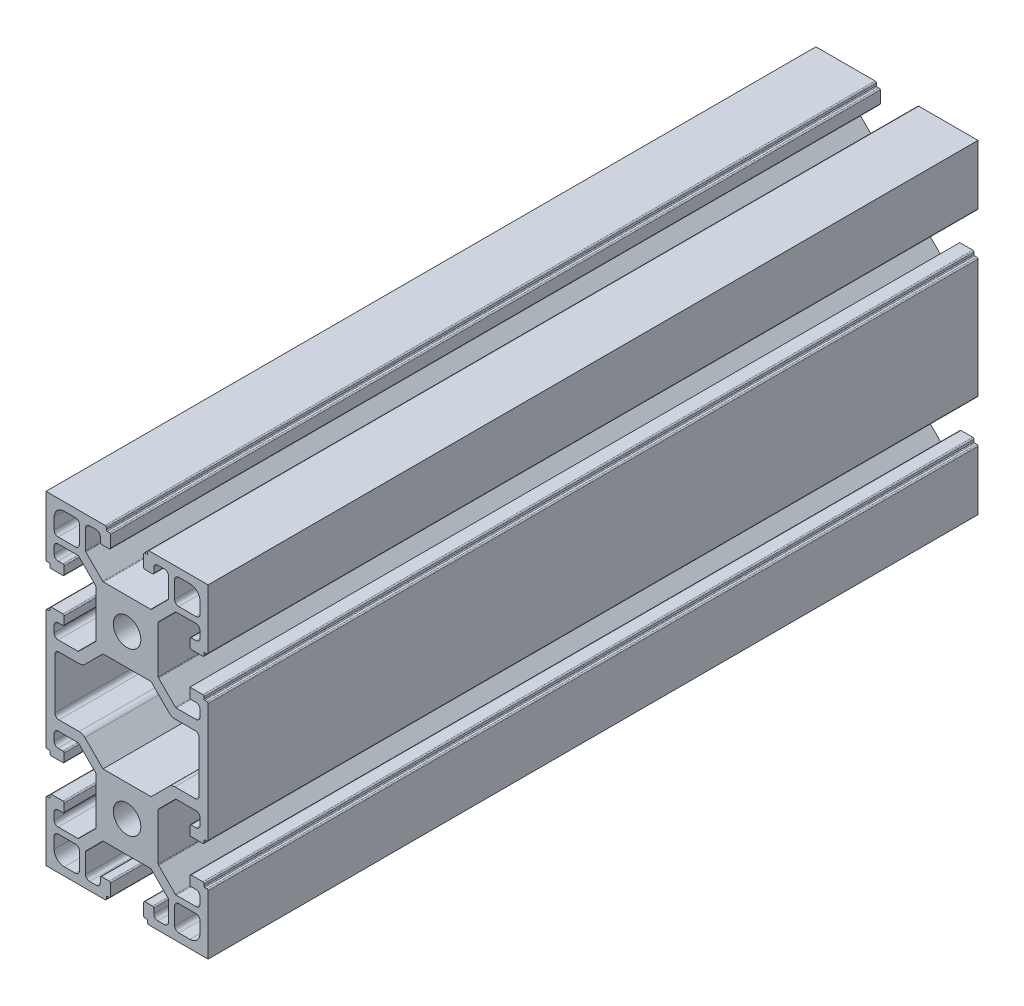
SolidWorks part; units mm, degrees
material "6061 合金"
ref_plane "前视基准面" through (0, 0, 0) normal (0, 0, 1) x (1, 0, 0)
ref_plane "上视基准面" through (0, 0, 0) normal (0, 1, 0) x (1, 0, 0)
ref_plane "右视基准面" through (0, 0, 0) normal (1, 0, 0) x (0, 0, -1)
sketch "Model" plane through (0, 0, 0) normal (0, 0, 1) x (1, 0, 0)
  line L0 (714.4099, 268.2298) -> (714.4099, 266.3298)
  line L1 (712.9099, 268.5298) -> (714.1099, 268.5298)
  line L2 (711.9099, 271.1798) -> (711.9099, 269.5298)
  line L3 (717.7679, 272.1798) -> (712.9099, 272.1798)
  line L4 (722.1221, 267.9499) -> (717.98, 272.0919)
  line L5 (722.2099, 256.1218) -> (722.2099, 267.7378)
  line L6 (717.98, 251.7677) -> (722.1221, 255.9097)
  line L7 (712.9099, 251.6798) -> (717.7679, 251.6798)
  line L8 (711.9099, 254.3298) -> (711.9099, 252.6798)
  line L9 (714.1099, 255.3298) -> (712.9099, 255.3298)
  line L10 (714.4099, 257.5298) -> (714.4099, 255.6298)
  line L11 (711.2099, 257.8298) -> (714.1099, 257.8298)
  line L12 (710.9099, 257.0298) -> (710.9099, 257.5298)
  line L13 (710.2099, 256.8298) -> (710.7099, 256.8298)
  line L14 (709.9099, 241.9298) -> (709.9099, 256.5298)
  line L15 (709.9099, 227.3298) -> (709.9099, 241.9298)
  line L16 (710.7099, 227.0298) -> (710.2099, 227.0298)
  line L17 (710.9099, 226.3298) -> (710.9099, 226.8298)
  line L18 (714.1099, 226.0298) -> (711.2099, 226.0298)
  line L19 (714.4099, 228.2298) -> (714.4099, 226.3298)
  line L20 (712.9099, 228.5298) -> (714.1099, 228.5298)
  line L21 (711.9099, 231.1798) -> (711.9099, 229.5298)
  line L22 (717.7679, 232.1798) -> (712.9099, 232.1798)
  line L23 (722.1221, 227.9499) -> (717.98, 232.0919)
  line L24 (722.2099, 216.1218) -> (722.2099, 227.7378)
  line L25 (717.98, 211.7677) -> (722.1221, 215.9097)
  line L26 (712.9099, 211.6798) -> (717.7679, 211.6798)
  line L27 (711.9099, 214.3298) -> (711.9099, 212.6798)
  line L28 (714.1099, 215.3298) -> (712.9099, 215.3298)
  line L29 (714.4099, 217.5298) -> (714.4099, 215.6298)
  line L30 (711.2099, 217.8298) -> (714.1099, 217.8298)
  line L31 (710.9099, 217.0298) -> (710.9099, 217.5298)
  line L32 (710.2099, 216.8298) -> (710.7099, 216.8298)
  line L33 (709.9099, 201.9298) -> (709.9099, 216.5298)
  line L34 (724.5099, 201.9298) -> (709.9099, 201.9298)
  line L35 (724.8099, 202.7298) -> (724.8099, 202.2298)
  line L36 (725.5099, 202.9298) -> (725.0099, 202.9298)
  line L37 (725.8099, 206.1298) -> (725.8099, 203.2298)
  line L38 (723.6099, 206.4298) -> (725.5099, 206.4298)
  line L39 (723.3099, 204.9298) -> (723.3099, 206.1298)
  line L40 (720.6599, 203.9298) -> (722.3099, 203.9298)
  line L41 (719.6599, 209.7878) -> (719.6599, 204.9298)
  line L42 (723.8898, 214.1419) -> (719.7478, 209.9999)
  line L43 (735.7179, 214.2298) -> (724.1019, 214.2298)
  line L44 (740.0721, 209.9999) -> (735.93, 214.1419)
  line L45 (740.1599, 204.9298) -> (740.1599, 209.7878)
  line L46 (737.5099, 203.9298) -> (739.1599, 203.9298)
  line L47 (736.5099, 206.1298) -> (736.5099, 204.9298)
  line L48 (734.3099, 206.4298) -> (736.2099, 206.4298)
  line L49 (734.0099, 203.2298) -> (734.0099, 206.1298)
  line L50 (734.8099, 202.9298) -> (734.3099, 202.9298)
  line L51 (735.0099, 202.2298) -> (735.0099, 202.7298)
  line L52 (749.9099, 201.9298) -> (735.3099, 201.9298)
  line L53 (749.9099, 216.5298) -> (749.9099, 201.9298)
  line L54 (749.1099, 216.8298) -> (749.6099, 216.8298)
  line L55 (748.9099, 217.5298) -> (748.9099, 217.0298)
  line L56 (745.7099, 217.8298) -> (748.6099, 217.8298)
  line L57 (745.4099, 215.6298) -> (745.4099, 217.5298)
  line L58 (746.9099, 215.3298) -> (745.7099, 215.3298)
  line L59 (747.9099, 212.6798) -> (747.9099, 214.3298)
  line L60 (742.0519, 211.6798) -> (746.9099, 211.6798)
  line L61 (737.6978, 215.9097) -> (741.8398, 211.7677)
  line L62 (737.6099, 227.7378) -> (737.6099, 216.1218)
  line L63 (741.8398, 232.0919) -> (737.6978, 227.9499)
  line L64 (746.9099, 232.1798) -> (742.0519, 232.1798)
  line L65 (747.9099, 229.5298) -> (747.9099, 231.1798)
  line L66 (745.7099, 228.5298) -> (746.9099, 228.5298)
  line L67 (745.4099, 226.3298) -> (745.4099, 228.2298)
  line L68 (748.6099, 226.0298) -> (745.7099, 226.0298)
  line L69 (748.9099, 226.8298) -> (748.9099, 226.3298)
  line L70 (749.6099, 227.0298) -> (749.1099, 227.0298)
  line L71 (749.9099, 241.9298) -> (749.9099, 227.3298)
  line L72 (749.9099, 256.5298) -> (749.9099, 241.9298)
  line L73 (749.1099, 256.8298) -> (749.6099, 256.8298)
  line L74 (748.9099, 257.5298) -> (748.9099, 257.0298)
  line L75 (745.4099, 257.8298) -> (748.6099, 257.8298)
  line L76 (745.4099, 255.3298) -> (745.4099, 257.8298)
  line L77 (746.9099, 255.3298) -> (745.4099, 255.3298)
  line L78 (747.9099, 252.6798) -> (747.9099, 254.3298)
  line L79 (742.0519, 251.6798) -> (746.9099, 251.6798)
  line L80 (737.6978, 255.9097) -> (741.8398, 251.7677)
  line L81 (737.6099, 267.7378) -> (737.6099, 256.1218)
  line L82 (741.8398, 272.0919) -> (737.6978, 267.9499)
  line L83 (746.9099, 272.1798) -> (742.0519, 272.1798)
  line L84 (747.9099, 269.5298) -> (747.9099, 271.1798)
  line L85 (745.7099, 268.5298) -> (746.9099, 268.5298)
  line L86 (745.4099, 266.3298) -> (745.4099, 268.2298)
  line L87 (748.6099, 266.0298) -> (745.7099, 266.0298)
  line L88 (748.9099, 266.8298) -> (748.9099, 266.3298)
  line L89 (749.6099, 267.0298) -> (749.1099, 267.0298)
  line L90 (749.9099, 281.9298) -> (749.9099, 267.3298)
  line L91 (735.3099, 281.9298) -> (749.9099, 281.9298)
  line L92 (735.0099, 281.1298) -> (735.0099, 281.6298)
  line L93 (734.3099, 280.9298) -> (734.8099, 280.9298)
  line L94 (734.0099, 277.7298) -> (734.0099, 280.6298)
  line L95 (736.2099, 277.4298) -> (734.3099, 277.4298)
  line L96 (736.5099, 278.9298) -> (736.5099, 277.7298)
  line L97 (739.1599, 279.9298) -> (737.5099, 279.9298)
  line L98 (740.1599, 274.0718) -> (740.1599, 278.9298)
  line L99 (735.93, 269.7177) -> (740.0721, 273.8597)
  line L100 (724.1019, 269.6298) -> (735.7179, 269.6298)
  line L101 (719.7478, 273.8597) -> (723.8898, 269.7177)
  line L102 (719.6599, 278.9298) -> (719.6599, 274.0718)
  line L103 (722.3099, 279.9298) -> (720.6599, 279.9298)
  line L104 (723.3099, 277.7298) -> (723.3099, 278.9298)
  line L105 (725.5099, 277.4298) -> (723.6099, 277.4298)
  line L106 (725.8099, 280.6298) -> (725.8099, 277.7298)
  line L107 (725.0099, 280.9298) -> (725.5099, 280.9298)
  line L108 (724.8099, 281.6298) -> (724.8099, 281.1298)
  line L109 (709.9099, 281.9298) -> (724.5099, 281.9298)
  line L110 (709.9099, 267.3298) -> (709.9099, 281.9298)
  line L111 (710.7099, 267.0298) -> (710.2099, 267.0298)
  line L112 (710.9099, 266.3298) -> (710.9099, 266.8298)
  line L113 (714.1099, 266.0298) -> (711.2099, 266.0298)
  line L114 (718.0993, 234.6798) -> (713.1099, 234.6798)
  line L115 (712.1099, 235.6798) -> (712.1099, 241.9298)
  line L116 (712.1099, 241.9298) -> (712.1099, 248.1798)
  line L117 (713.1099, 249.1798) -> (718.0993, 249.1798)
  line L118 (719.5135, 249.7656) -> (723.9777, 254.2298)
  line L119 (723.9777, 254.2298) -> (735.8422, 254.2298)
  line L120 (735.8422, 254.2298) -> (740.3064, 249.7656)
  line L121 (741.7206, 249.1798) -> (746.7099, 249.1798)
  line L122 (747.7099, 248.1798) -> (747.7099, 241.9298)
  line L123 (747.7099, 241.9298) -> (747.7099, 235.6798)
  line L124 (746.7099, 234.6798) -> (741.7206, 234.6798)
  line L125 (740.3064, 234.094) -> (735.8422, 229.6298)
  line L126 (735.8422, 229.6298) -> (723.9777, 229.6298)
  line L127 (723.9777, 229.6298) -> (719.5135, 234.094)
  line L128 (718.1599, 278.9298) -> (718.1599, 274.6798)
  line L129 (717.1599, 273.6798) -> (712.9099, 273.6798)
  line L130 (711.9099, 274.6798) -> (711.9099, 277.4298)
  line L131 (714.4099, 279.9298) -> (717.1599, 279.9298)
  line L132 (741.6599, 278.9298) -> (741.6599, 274.6798)
  line L133 (742.6599, 273.6798) -> (746.9099, 273.6798)
  line L134 (747.9099, 274.6798) -> (747.9099, 277.4298)
  line L135 (745.4099, 279.9298) -> (742.6599, 279.9298)
  line L136 (711.9099, 206.4298) -> (711.9099, 209.1798)
  line L137 (712.9099, 210.1798) -> (717.1599, 210.1798)
  line L138 (718.1599, 209.1798) -> (718.1599, 204.9298)
  line L139 (717.1599, 203.9298) -> (714.4099, 203.9298)
  line L140 (742.6599, 203.9298) -> (745.4099, 203.9298)
  line L141 (747.9099, 206.4298) -> (747.9099, 209.1798)
  line L142 (746.9099, 210.1798) -> (742.6599, 210.1798)
  line L143 (741.6599, 209.1798) -> (741.6599, 204.9298)
  arc A0 (714.1099, 266.0298) -> (714.4099, 266.3298) centre (714.1099, 266.3298) ccw
  arc A1 (714.4099, 268.2298) -> (714.1099, 268.5298) centre (714.1099, 268.2298) ccw
  arc A2 (711.9099, 269.5298) -> (712.9099, 268.5298) centre (712.9099, 269.5298) ccw
  arc A3 (712.9099, 272.1798) -> (711.9099, 271.1798) centre (712.9099, 271.1798) ccw
  arc A4 (717.98, 272.0919) -> (717.7679, 272.1798) centre (717.7679, 271.8798) ccw
  arc A5 (722.2099, 267.7378) -> (722.1221, 267.9499) centre (721.9099, 267.7378) ccw
  arc A6 (722.1221, 255.9097) -> (722.2099, 256.1218) centre (721.9099, 256.1218) ccw
  arc A7 (717.7679, 251.6798) -> (717.98, 251.7677) centre (717.7679, 251.9798) ccw
  arc A8 (711.9099, 252.6798) -> (712.9099, 251.6798) centre (712.9099, 252.6798) ccw
  arc A9 (712.9099, 255.3298) -> (711.9099, 254.3298) centre (712.9099, 254.3298) ccw
  arc A10 (714.1099, 255.3298) -> (714.4099, 255.6298) centre (714.1099, 255.6298) ccw
  arc A11 (714.4099, 257.5298) -> (714.1099, 257.8298) centre (714.1099, 257.5298) ccw
  arc A12 (711.2099, 257.8298) -> (710.9099, 257.5298) centre (711.2099, 257.5298) ccw
  arc A13 (710.7099, 256.8298) -> (710.9099, 257.0298) centre (710.7099, 257.0298) ccw
  arc A14 (710.2099, 256.8298) -> (709.9099, 256.5298) centre (710.2099, 256.5298) ccw
  arc A15 (709.9099, 227.3298) -> (710.2099, 227.0298) centre (710.2099, 227.3298) ccw
  arc A16 (710.9099, 226.8298) -> (710.7099, 227.0298) centre (710.7099, 226.8298) ccw
  arc A17 (710.9099, 226.3298) -> (711.2099, 226.0298) centre (711.2099, 226.3298) ccw
  arc A18 (714.1099, 226.0298) -> (714.4099, 226.3298) centre (714.1099, 226.3298) ccw
  arc A19 (714.4099, 228.2298) -> (714.1099, 228.5298) centre (714.1099, 228.2298) ccw
  arc A20 (711.9099, 229.5298) -> (712.9099, 228.5298) centre (712.9099, 229.5298) ccw
  arc A21 (712.9099, 232.1798) -> (711.9099, 231.1798) centre (712.9099, 231.1798) ccw
  arc A22 (717.98, 232.0919) -> (717.7679, 232.1798) centre (717.7679, 231.8798) ccw
  arc A23 (722.2099, 227.7378) -> (722.1221, 227.9499) centre (721.9099, 227.7378) ccw
  arc A24 (722.1221, 215.9097) -> (722.2099, 216.1218) centre (721.9099, 216.1218) ccw
  arc A25 (717.7679, 211.6798) -> (717.98, 211.7677) centre (717.7679, 211.9798) ccw
  arc A26 (711.9099, 212.6798) -> (712.9099, 211.6798) centre (712.9099, 212.6798) ccw
  arc A27 (712.9099, 215.3298) -> (711.9099, 214.3298) centre (712.9099, 214.3298) ccw
  arc A28 (714.1099, 215.3298) -> (714.4099, 215.6298) centre (714.1099, 215.6298) ccw
  arc A29 (714.4099, 217.5298) -> (714.1099, 217.8298) centre (714.1099, 217.5298) ccw
  arc A30 (711.2099, 217.8298) -> (710.9099, 217.5298) centre (711.2099, 217.5298) ccw
  arc A31 (710.7099, 216.8298) -> (710.9099, 217.0298) centre (710.7099, 217.0298) ccw
  arc A32 (710.2099, 216.8298) -> (709.9099, 216.5298) centre (710.2099, 216.5298) ccw
  arc A34 (724.5099, 201.9298) -> (724.8099, 202.2298) centre (724.5099, 202.2298) ccw
  arc A35 (725.0099, 202.9298) -> (724.8099, 202.7298) centre (725.0099, 202.7298) ccw
  arc A36 (725.5099, 202.9298) -> (725.8099, 203.2298) centre (725.5099, 203.2298) ccw
  arc A37 (725.8099, 206.1298) -> (725.5099, 206.4298) centre (725.5099, 206.1298) ccw
  arc A38 (723.6099, 206.4298) -> (723.3099, 206.1298) centre (723.6099, 206.1298) ccw
  arc A39 (722.3099, 203.9298) -> (723.3099, 204.9298) centre (722.3099, 204.9298) ccw
  arc A40 (719.6599, 204.9298) -> (720.6599, 203.9298) centre (720.6599, 204.9298) ccw
  arc A41 (719.7478, 209.9999) -> (719.6599, 209.7878) centre (719.9599, 209.7878) ccw
  arc A42 (724.1019, 214.2298) -> (723.8898, 214.1419) centre (724.1019, 213.9298) ccw
  arc A43 (735.93, 214.1419) -> (735.7179, 214.2298) centre (735.7179, 213.9298) ccw
  arc A44 (740.1599, 209.7878) -> (740.0721, 209.9999) centre (739.8599, 209.7878) ccw
  arc A45 (739.1599, 203.9298) -> (740.1599, 204.9298) centre (739.1599, 204.9298) ccw
  arc A46 (736.5099, 204.9298) -> (737.5099, 203.9298) centre (737.5099, 204.9298) ccw
  arc A47 (736.5099, 206.1298) -> (736.2099, 206.4298) centre (736.2099, 206.1298) ccw
  arc A48 (734.3099, 206.4298) -> (734.0099, 206.1298) centre (734.3099, 206.1298) ccw
  arc A49 (734.0099, 203.2298) -> (734.3099, 202.9298) centre (734.3099, 203.2298) ccw
  arc A50 (735.0099, 202.7298) -> (734.8099, 202.9298) centre (734.8099, 202.7298) ccw
  arc A51 (735.0099, 202.2298) -> (735.3099, 201.9298) centre (735.3099, 202.2298) ccw
  arc A53 (749.9099, 216.5298) -> (749.6099, 216.8298) centre (749.6099, 216.5298) ccw
  arc A54 (748.9099, 217.0298) -> (749.1099, 216.8298) centre (749.1099, 217.0298) ccw
  arc A55 (748.9099, 217.5298) -> (748.6099, 217.8298) centre (748.6099, 217.5298) ccw
  arc A56 (745.7099, 217.8298) -> (745.4099, 217.5298) centre (745.7099, 217.5298) ccw
  arc A57 (745.4099, 215.6298) -> (745.7099, 215.3298) centre (745.7099, 215.6298) ccw
  arc A58 (747.9099, 214.3298) -> (746.9099, 215.3298) centre (746.9099, 214.3298) ccw
  arc A59 (746.9099, 211.6798) -> (747.9099, 212.6798) centre (746.9099, 212.6798) ccw
  arc A60 (741.8398, 211.7677) -> (742.0519, 211.6798) centre (742.0519, 211.9798) ccw
  arc A61 (737.6099, 216.1218) -> (737.6978, 215.9097) centre (737.9099, 216.1218) ccw
  arc A62 (737.6978, 227.9499) -> (737.6099, 227.7378) centre (737.9099, 227.7378) ccw
  arc A63 (742.0519, 232.1798) -> (741.8398, 232.0919) centre (742.0519, 231.8798) ccw
  arc A64 (747.9099, 231.1798) -> (746.9099, 232.1798) centre (746.9099, 231.1798) ccw
  arc A65 (746.9099, 228.5298) -> (747.9099, 229.5298) centre (746.9099, 229.5298) ccw
  arc A66 (745.7099, 228.5298) -> (745.4099, 228.2298) centre (745.7099, 228.2298) ccw
  arc A67 (745.4099, 226.3298) -> (745.7099, 226.0298) centre (745.7099, 226.3298) ccw
  arc A68 (748.6099, 226.0298) -> (748.9099, 226.3298) centre (748.6099, 226.3298) ccw
  arc A69 (749.1099, 227.0298) -> (748.9099, 226.8298) centre (749.1099, 226.8298) ccw
  arc A70 (749.6099, 227.0298) -> (749.9099, 227.3298) centre (749.6099, 227.3298) ccw
  arc A71 (749.9099, 256.5298) -> (749.6099, 256.8298) centre (749.6099, 256.5298) ccw
  arc A72 (748.9099, 257.0298) -> (749.1099, 256.8298) centre (749.1099, 257.0298) ccw
  arc A73 (748.9099, 257.5298) -> (748.6099, 257.8298) centre (748.6099, 257.5298) ccw
  arc A74 (747.9099, 254.3298) -> (746.9099, 255.3298) centre (746.9099, 254.3298) ccw
  arc A75 (746.9099, 251.6798) -> (747.9099, 252.6798) centre (746.9099, 252.6798) ccw
  arc A76 (741.8398, 251.7677) -> (742.0519, 251.6798) centre (742.0519, 251.9798) ccw
  arc A77 (737.6099, 256.1218) -> (737.6978, 255.9097) centre (737.9099, 256.1218) ccw
  arc A78 (737.6978, 267.9499) -> (737.6099, 267.7378) centre (737.9099, 267.7378) ccw
  arc A79 (742.0519, 272.1798) -> (741.8398, 272.0919) centre (742.0519, 271.8798) ccw
  arc A80 (747.9099, 271.1798) -> (746.9099, 272.1798) centre (746.9099, 271.1798) ccw
  arc A81 (746.9099, 268.5298) -> (747.9099, 269.5298) centre (746.9099, 269.5298) ccw
  arc A82 (745.7099, 268.5298) -> (745.4099, 268.2298) centre (745.7099, 268.2298) ccw
  arc A83 (745.4099, 266.3298) -> (745.7099, 266.0298) centre (745.7099, 266.3298) ccw
  arc A84 (748.6099, 266.0298) -> (748.9099, 266.3298) centre (748.6099, 266.3298) ccw
  arc A85 (749.1099, 267.0298) -> (748.9099, 266.8298) centre (749.1099, 266.8298) ccw
  arc A86 (749.6099, 267.0298) -> (749.9099, 267.3298) centre (749.6099, 267.3298) ccw
  arc A88 (735.3099, 281.9298) -> (735.0099, 281.6298) centre (735.3099, 281.6298) ccw
  arc A89 (734.8099, 280.9298) -> (735.0099, 281.1298) centre (734.8099, 281.1298) ccw
  arc A90 (734.3099, 280.9298) -> (734.0099, 280.6298) centre (734.3099, 280.6298) ccw
  arc A91 (734.0099, 277.7298) -> (734.3099, 277.4298) centre (734.3099, 277.7298) ccw
  arc A92 (736.2099, 277.4298) -> (736.5099, 277.7298) centre (736.2099, 277.7298) ccw
  arc A93 (737.5099, 279.9298) -> (736.5099, 278.9298) centre (737.5099, 278.9298) ccw
  arc A94 (740.1599, 278.9298) -> (739.1599, 279.9298) centre (739.1599, 278.9298) ccw
  arc A95 (740.0721, 273.8597) -> (740.1599, 274.0718) centre (739.8599, 274.0718) ccw
  arc A96 (735.7179, 269.6298) -> (735.93, 269.7177) centre (735.7179, 269.9298) ccw
  arc A97 (723.8898, 269.7177) -> (724.1019, 269.6298) centre (724.1019, 269.9298) ccw
  arc A98 (719.6599, 274.0718) -> (719.7478, 273.8597) centre (719.9599, 274.0718) ccw
  arc A99 (720.6599, 279.9298) -> (719.6599, 278.9298) centre (720.6599, 278.9298) ccw
  arc A100 (723.3099, 278.9298) -> (722.3099, 279.9298) centre (722.3099, 278.9298) ccw
  arc A101 (723.3099, 277.7298) -> (723.6099, 277.4298) centre (723.6099, 277.7298) ccw
  arc A102 (725.5099, 277.4298) -> (725.8099, 277.7298) centre (725.5099, 277.7298) ccw
  arc A103 (725.8099, 280.6298) -> (725.5099, 280.9298) centre (725.5099, 280.6298) ccw
  arc A104 (724.8099, 281.1298) -> (725.0099, 280.9298) centre (725.0099, 281.1298) ccw
  arc A105 (724.8099, 281.6298) -> (724.5099, 281.9298) centre (724.5099, 281.6298) ccw
  arc A107 (709.9099, 267.3298) -> (710.2099, 267.0298) centre (710.2099, 267.3298) ccw
  arc A108 (710.9099, 266.8298) -> (710.7099, 267.0298) centre (710.7099, 266.8298) ccw
  arc A109 (710.9099, 266.3298) -> (711.2099, 266.0298) centre (711.2099, 266.3298) ccw
  arc A110 (712.1099, 235.6798) -> (713.1099, 234.6798) centre (713.1099, 235.6798) ccw
  arc A111 (713.1099, 249.1798) -> (712.1099, 248.1798) centre (713.1099, 248.1798) ccw
  arc A112 (718.0993, 249.1798) -> (719.5135, 249.7656) centre (718.0993, 251.1798) ccw
  arc A113 (740.3064, 249.7656) -> (741.7206, 249.1798) centre (741.7206, 251.1798) ccw
  arc A114 (747.7099, 248.1798) -> (746.7099, 249.1798) centre (746.7099, 248.1798) ccw
  arc A115 (746.7099, 234.6798) -> (747.7099, 235.6798) centre (746.7099, 235.6798) ccw
  arc A116 (741.7206, 234.6798) -> (740.3064, 234.094) centre (741.7206, 232.6798) ccw
  arc A117 (719.5135, 234.094) -> (718.0993, 234.6798) centre (718.0993, 232.6798) ccw
  circle A118 centre (729.9099, 261.9298) radius 3.4
  arc A119 (718.1599, 278.9298) -> (717.1599, 279.9298) centre (717.1599, 278.9298) ccw
  arc A120 (717.1599, 273.6798) -> (718.1599, 274.6798) centre (717.1599, 274.6798) ccw
  arc A121 (711.9099, 274.6798) -> (712.9099, 273.6798) centre (712.9099, 274.6798) ccw
  arc A122 (714.4099, 279.9298) -> (711.9099, 277.4298) centre (714.4099, 277.4298) ccw
  arc A123 (742.6599, 279.9298) -> (741.6599, 278.9298) centre (742.6599, 278.9298) ccw
  arc A124 (741.6599, 274.6798) -> (742.6599, 273.6798) centre (742.6599, 274.6798) ccw
  arc A125 (746.9099, 273.6798) -> (747.9099, 274.6798) centre (746.9099, 274.6798) ccw
  arc A126 (747.9099, 277.4298) -> (745.4099, 279.9298) centre (745.4099, 277.4298) ccw
  circle A127 centre (729.9099, 221.9298) radius 3.4
  arc A128 (712.9099, 210.1798) -> (711.9099, 209.1798) centre (712.9099, 209.1798) ccw
  arc A129 (718.1599, 209.1798) -> (717.1599, 210.1798) centre (717.1599, 209.1798) ccw
  arc A130 (717.1599, 203.9298) -> (718.1599, 204.9298) centre (717.1599, 204.9298) ccw
  arc A131 (711.9099, 206.4298) -> (714.4099, 203.9298) centre (714.4099, 206.4298) ccw
  arc A132 (741.6599, 204.9298) -> (742.6599, 203.9298) centre (742.6599, 204.9298) ccw
  arc A133 (745.4099, 203.9298) -> (747.9099, 206.4298) centre (745.4099, 206.4298) ccw
  arc A134 (747.9099, 209.1798) -> (746.9099, 210.1798) centre (746.9099, 209.1798) ccw
  arc A135 (742.6599, 210.1798) -> (741.6599, 209.1798) centre (742.6599, 209.1798) ccw
extrude "凸台-拉伸1" add sketch "Model" along normal mid plane 190
cosmetic thread "孔螺蚊线1" parameters "D1"=16, "D2"=8
cosmetic thread "孔螺蚊线2" parameters "D1"=16, "D2"=8
cosmetic thread "孔螺蚊线3" parameters "D1"=16, "D2"=8
cosmetic thread "孔螺蚊线4" parameters "D1"=16, "D2"=8
hole_wizard "M8 螺纹孔1" positions "3D草图1" profile "草图2" tap size "M8" standard "GB"
sketch3d "3D草图1"
  line L0 (729.9099, 261.9298, 95) -> (729.9099, 261.9298, -95) construction
  line L1 (729.9099, 221.9298, 95) -> (729.9099, 221.9298, -95) construction
  point P0 (729.9099, 261.9298, 95)
  point P4 (729.9099, 221.9298, 95)
  point P10 (729.9099, 221.9298, -95)
  point P12 (729.9099, 261.9298, -95)
sketch "草图2" plane through (729.9099, 261.9298, 95) normal (1, 0, 0) x (0, -1, 0)
  line L0 (0, 0) -> (0, 21.7929)
  line L1 (0, 21.7929) -> (3.4, 19.75)
  line L2 (3.4, 19.75) -> (3.4, 0)
  line L5 (3.4, 0) -> (0, 0)
  line L10 (0, 21.7929) -> (-3.4, 19.75) construction
  line L11 (0, -6.35) -> (0, 107.95) construction
  dimension "螺纹孔钻头直径" = 6.8
  dimension "螺纹孔钻头深度" = 19.75
  dimension "导头角度" = 118
